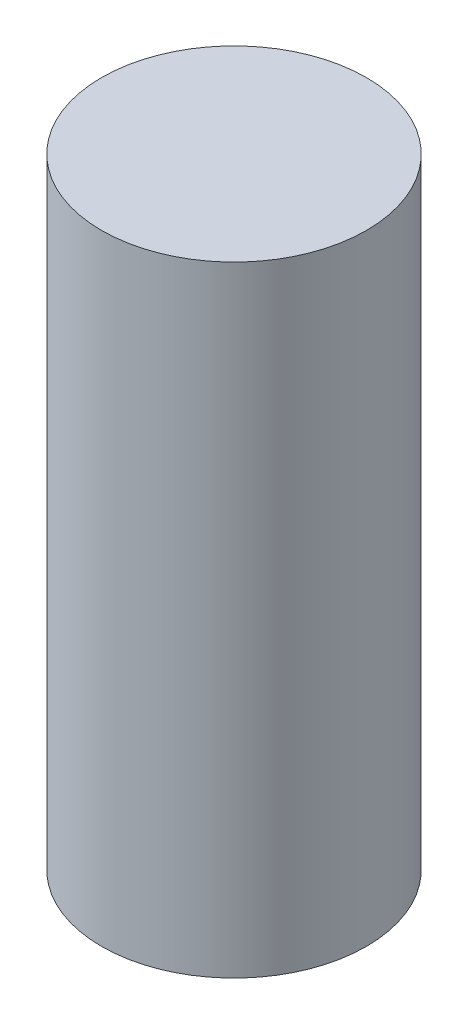
SolidWorks part; units mm, degrees
material "尼龙"
ref_plane "Front Plane" through (0, 0, 0) normal (0, 0, 1) x (1, 0, 0)
ref_plane "Top Plane" through (0, 0, 0) normal (0, 1, 0) x (1, 0, 0)
ref_plane "Right Plane" through (0, 0, 0) normal (1, 0, 0) x (0, 0, -1)
sketch "Sketch1" plane through (0, 0, 0) normal (0, 1, 0) x (1, 0, 0)
  circle A0 centre (0, 0) radius 35
  dimension "D1" = 70
extrude "Boss-Extrude1" add sketch "Sketch1" along normal blind 163.9
